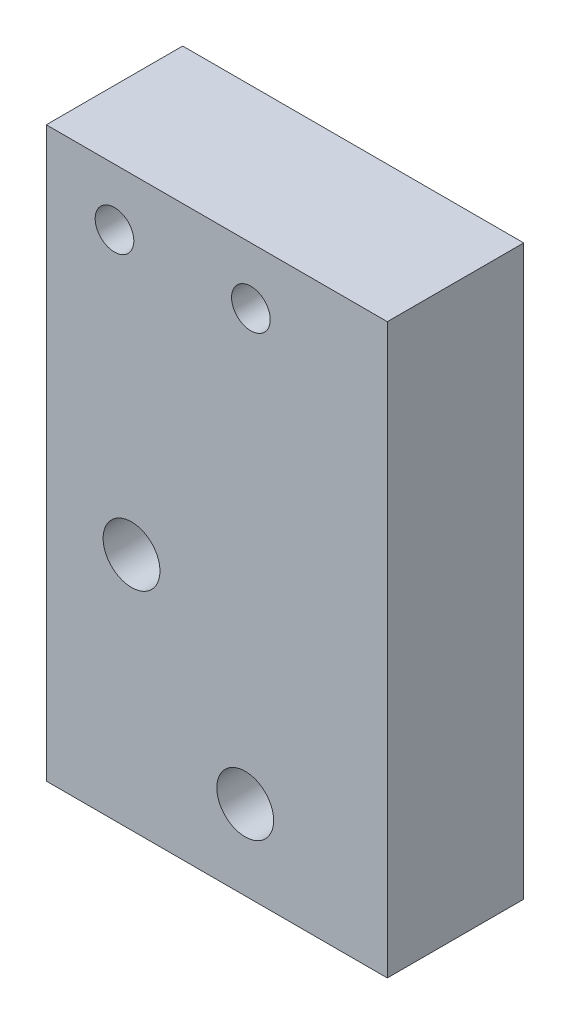
from build123d import *

# Parameters (mm, degrees)
SKETCH_1_W                                         = 30
SKETCH_1_H                                         = 50
BOSS_EXTRUDE_1_DEPTH                               = 12
M6_TAPPED_HOLE_1_D                                 = 5
M3_SOCKET_HEAD_CAP_SCREW_COUNTERBORE_1_D           = 3.4
M3_SOCKET_HEAD_CAP_SCREW_COUNTERBORE_1_CBORE_D     = 6.5
M3_SOCKET_HEAD_CAP_SCREW_COUNTERBORE_1_CBORE_DEPTH = 3
LINEAR_PATTERN_1_COUNT                             = 2
LINEAR_PATTERN_1_PITCH                             = 12


with BuildPart() as part:
    # Sketch 1 → Boss-Extrude 1 (new body)
    with BuildSketch(Plane.XY):
        Rectangle(SKETCH_1_W, SKETCH_1_H)
    extrude(amount=BOSS_EXTRUDE_1_DEPTH)

    # M6 Tapped Hole 1 (through all)
    with Locations(Plane(origin=(0, 0, 0), x_dir=(-1, 0, 0), z_dir=(0, 0, -1))):
        with Locations((7.5, -4), (-2.5, -18)):
            Hole(M6_TAPPED_HOLE_1_D / 2)

    # M3 Socket Head Cap Screw Counterbore 1 (through all)
    with Locations(Plane(origin=(0, 0, 0), x_dir=(-1, 0, 0), z_dir=(0, 0, -1))):
        with Locations((9, 20)):
            m3_socket_head_cap_screw_counterbore_1 = CounterBoreHole(M3_SOCKET_HEAD_CAP_SCREW_COUNTERBORE_1_D / 2, M3_SOCKET_HEAD_CAP_SCREW_COUNTERBORE_1_CBORE_D / 2, M3_SOCKET_HEAD_CAP_SCREW_COUNTERBORE_1_CBORE_DEPTH)

    # Linear Pattern 1: M3 Socket Head Cap Screw Counterbore 1 ×2
    with Locations(*[(i * LINEAR_PATTERN_1_PITCH, 0, 0) for i in range(1, LINEAR_PATTERN_1_COUNT)]):
        add(m3_socket_head_cap_screw_counterbore_1, mode=Mode.SUBTRACT)


solid = part.part
